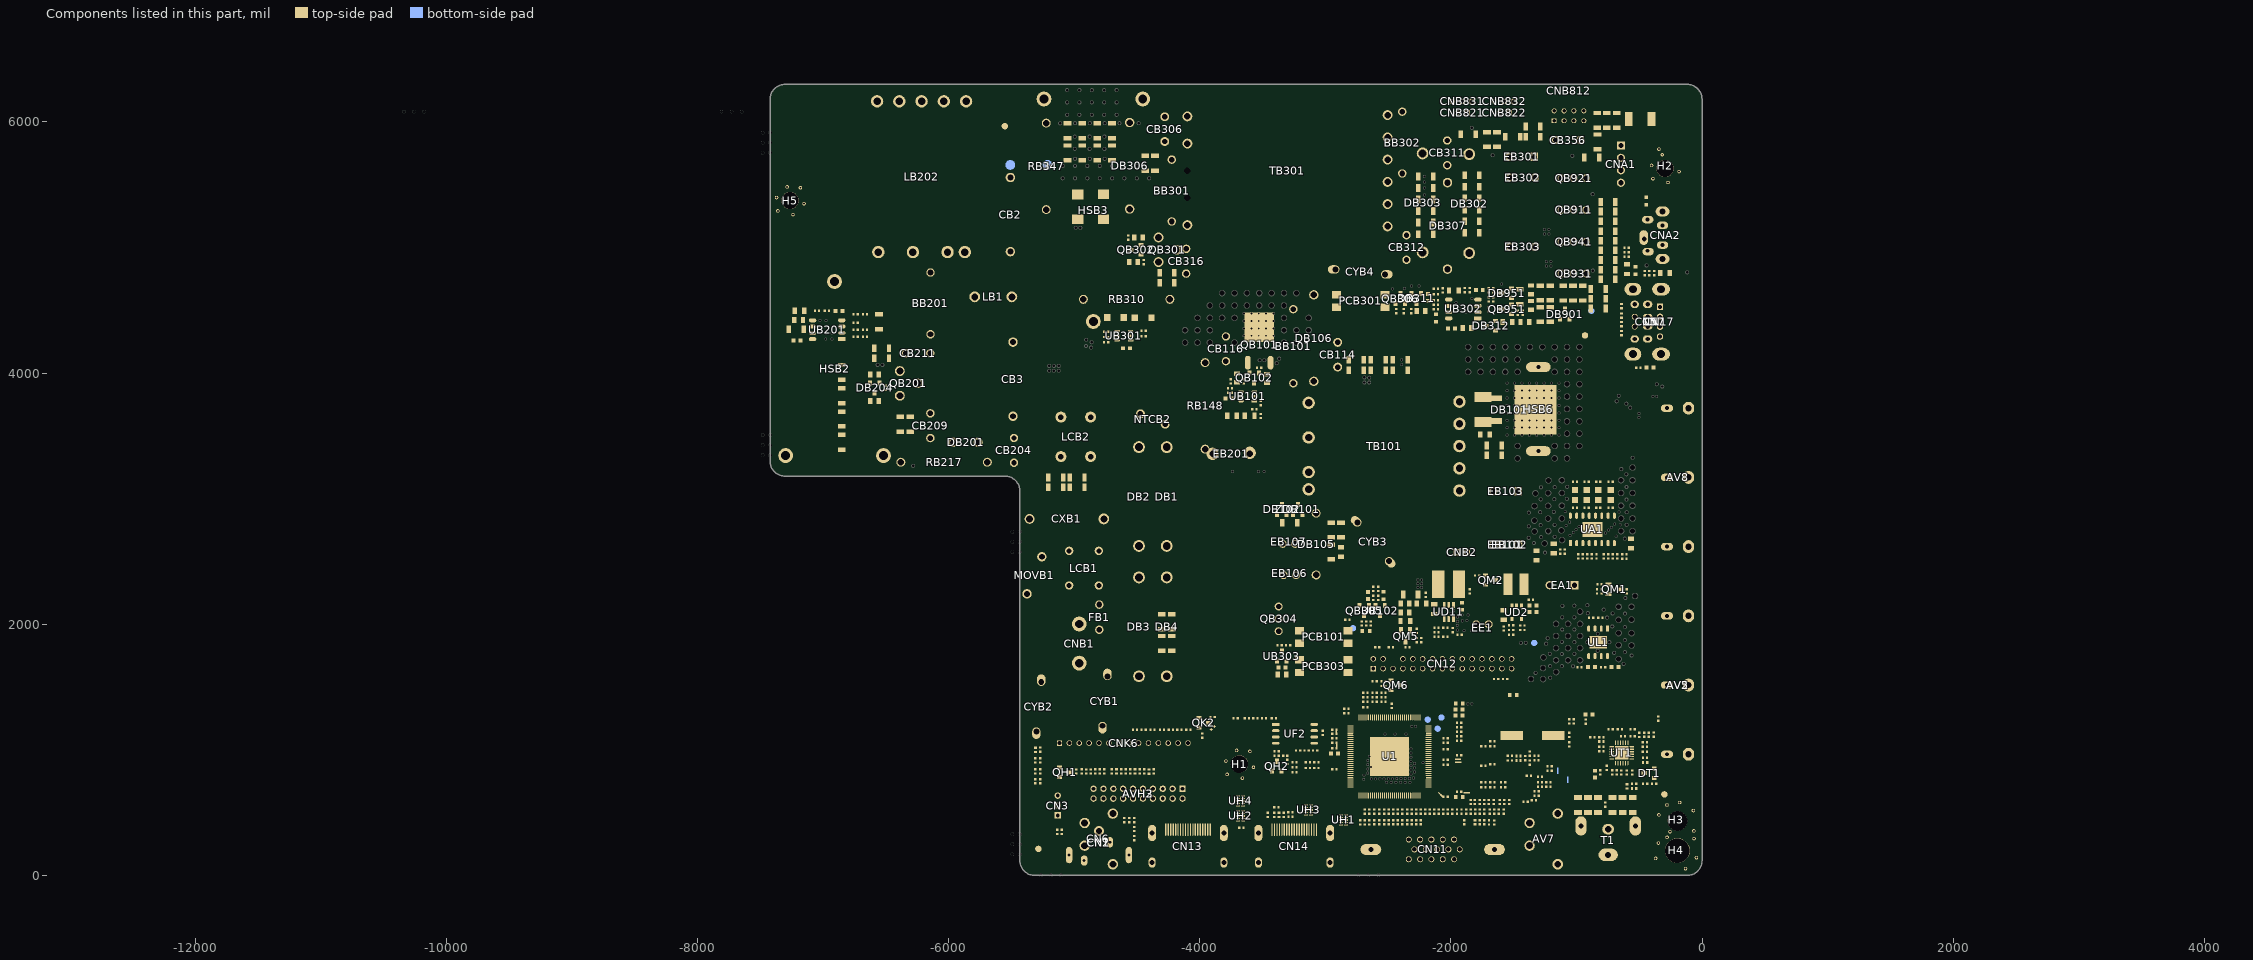
[diagram p0: the components of this part, seen from the top]
# Altium PCB MISC84277.PcbDoc (part 15 of 15)
Units mil, origin at the board's own origin, x right, y up, seen from the top; angles counter-clockwise.
Board outline 7422.08 x 6299.21 mil, 2 copper layers (TopLayer, BottomLayer), stack 61.855 mil thick; 709 components, 395 nets, 2812 pads, 811 vias.

## Silkscreen, mask and mechanical layers (free items; w line width, h text height)
TopOverlay:
  drawing of 481 lines, arcs and shapes, not listed
  text "LED DRIVER" at -855.43,6223.54 h60
  text "Solder Mask:" at 948.13,5998.57 h60
  text "IPC SM-840" at 1360.63,5997.57 h60
  text "Silkscreen Color:" at 2126.63,5997.57 h60
  text "White" at 2605.63,5997.57 h60
  text "Units:" at 2126.63,5898.57 h60
  text "PTH Copper Thickness:" at 948.13,5897.57 h60
  text "mm" at 2324.63,5897.07 h60
  text ">20um" at 1621.63,5896.57 h60
  text "4.2 --- 4.6" at 2127.29,5799.1 h60
  text "Dielectric Constant Er@1GHz To 1MHz:" at 947.79,5798.6 h60
  text "Panel Size:" at 946.13,5700.07 h60
  text "2L,2,164.00×165.50mm,FR4(TG130-CTI175),1OZ,Green,OSP,1.2mm" at 1251.29,5700.1 h60
  text "Silkscreen on PTH:" at 946.63,5598.57 h60
  text "Primary Side Retained;" at 1464.63,5597.57 h60
  text "Secondary Side  Removed for Soldering" at 2126.63,5596.07 h60
  text "Special Requirements" at 945.62,5507.89 h60
  text "If engineering questions get no reply within 2 hours, call: PHONE_A" at 2832.29,5500.6 h60
  text "SPEAKER" at -803.98,5452.5 h50 r90
  text "1. Lead-free hot air leveling (HAL_LF, Lead Free Hot Air Leveling)" at 1536.51,5404.3 h60
  text "2. Organic solderability preservative (OSP, Organic Solderability Preservatives)" at 1536.51,5320.3 h60
  text "3. Electroless nickel immersion gold (ENIG, Electroless Nickel/Immersion Gold)" at 1535.01,5228.8 h60
  text "Plated Technics" at 1020.63,5194.07 h60
  text "4. Electroless nickel immersion gold + gold finger (ENIG_G/F, Electroless Nickel/Immersion Gold + Gold Finger)" at 1536.51,5148.3 h60
  text "5. Gold plated (Gold_plated, Gold-plated)" at 1537.51,5067.8 h60
  text "6. Gold plated + gold finger (Gold_Plated_G/F, Gold-plated + Gold Finger)" at 1538.01,4989.8 h60
  text "Impedance Control" at 950.36,4761.21 h60
  text "Target Impedance" at 1747.19,4761.31 h60
  text "Width & Clearance" at 2493.02,4761.08 h60
  text "Layer(s)" at 3261.33,4761.39 h60
  text "75 +/- 10% Ohm" at 1769.39,4660.61 h60
  text "G/12/15.8/12/G mil" at 2450.44,4659.93 h60
  text "layer 1" at 3261.33,4660.05 h60
  text "Single End Impedance" at 950.36,4614.39 h60
  text "[ Zo ]" at 1173.86,4477.14 h60
  text "2" at -12847.94,4319.68 h160 r270
  text "G/5/7/5/7/5/G mil" at 2450.94,4263.43 h60
  text "100 +/- 10% Ohm" at 1746.89,4262.42 h60
  text "layer 1" at 3262.82,4260.64 h60
  text "Differential Impedance" at 950.22,4212.81 h60
  text "[ Zo ]" at 1173.35,4089.48 h60
  text "90 +/- 10% Ohm" at 1772.94,4064.43 h60
  text "layer 1" at 3258.82,4063.64 h60
  text "G/5/11/5/11/5/G mil" at 2450.94,4060.93 h60
  text "EXT-USB" at -281.5,4033.46 h60
  text "( G: Ground )" at 1083.43,3981.98 h60
  text "Common Mode Impedance" at 930,3760.3 h60
  text "[ Zc ]" at 1178,3679.3 h60
  text "Gerber Documents  .GTP&.GBP are used for making stencil" at 1842.55,3415.11 h60
  text "Stencil" at 943.42,3314.43 h60
  text "The same as XXXXXXXXXXXXX XXXXXX" at 1837.45,3222.78 h60
  text "Test jig" at 942.36,3122.45 h60
  text "The same as XXXXXXXXXXXXX XXXXXX" at 1838.45,3122.23 h60
  text "Wave-soldering jig" at 944.57,3024.21 h60
  text "The same as XXXXXXXXXXXXX XXXXXX" at 1840.35,3022.23 h60
  text "Solder paste" at 1842.55,2922.43 h60
  text "Production process" at 943.05,2920.93 h60
  text "Special Requirements" at 944.05,2822.93 h60
  text "Package Attention" at 943.43,2725.38 h60
  text "PWR UPGRADE" at -2224.9,2703.31 h60
  text "[Fragile components]" at 1179.66,2640.56 h60
  text "Footprint Matching" at 943.43,2525.38 h60
  text "GND" at -2144.95,2441.61 h50
  text "12V" at -1782,2438.93 h50
  text "[New component footprint]" at 1156.42,2437.43 h60
  text "Layer Stack Up Detail for" at 1084.39,2099.57 h100
  text ".Pcb_File_Name_No_Path" at 2145.21,2099.57 h100
  text "Layer" at 1248.75,1951.84 h50
  text "Gerber" at 1620.46,1951.84 h50
  text "Layer" at 1931.61,1951.84 h50
  text "Layer" at 2567.85,1951.84 h50
  text "Copper" at 3356.75,1951.84 h50
  text "Dielectric" at 3668.53,1951.84 h50
  text "Name" at 1248.75,1899.46 h50
  text "Document" at 1620.46,1899.46 h50
  text "Ordor" at 1931.61,1899.46 h50
  text "Stack up" at 2567.85,1899.46 h50
  text "Thickness" at 3356.75,1899.46 h50
  text "Height" at 3668.53,1899.46 h50
  text "1" at -67,1763 h160 r90
  text "TopOverlay" at 1248.45,1666.61 h60
  text ".GTO" at 1658.02,1664.05 h60
  text "T3.15AL 250V~" at -4651.2,1655.5 h78.74 r90
  text "0.4mil" at 3665.85,1579.02 h60
  text "LVDS" at -2202.76,1535.43 h60
  text "1" at 1984.81,1475.87 h60
  text "1.4mil" at 3369.81,1475.81 h60
  text "2" at 1984.87,1262.83 h60
  text "1.4mil" at 3368.1,1261.82 h60
  text "0.4mil" at 3668.52,1167.14 h60
  text "IR&KEY" at -4140.7,871.8 h60
  text "Notes:" at 920.32,604.26 h80
  text "1. No Plated Through Hole  overlap each other should be combined ,Residues between them should be eliminated." at 919.45,516.35 h60
  text "EXT-HDMI" at -4407.2,458 h55
  text "EXT-LINE OUT" at -4961,448.8 h55 r90
  text "2. Plated Through Hole superposition should be made as a bigger one." at 919.39,440.25 h60
  text "3. When there is not enough space for UL authentication marking,Manufacturer ID code and the Bar Code frame," at 919.45,371.75 h60
  text "only the Manufacturer  ID code is needed and layed wherever it can be." at 977.83,301.06 h60
  text "4. Spacing between two pads of IC package should be covered with solder oil." at 919.45,224.29 h60
  text "5. All trace should be covered with green oil unless otherwise specified. If discovers unusually, please confirm with us." at 919.45,150.88 h60
  text "6. Silkscreen overlaped SMD pads should be removed directly." at 919.45,77.57 h60
  text "7. The width of Carbon Sprayed must be 16mil wider than its trace." at 919.45,6.53 h60
  text "8. Bridging Thickness of V-cut  should be kept within 0.3±0.1mm when the width of single piece bare board is smaller than 20mm." at 919.45,-67.9 h60
  text "9. There is no need to plugged with green oil when the diameter of vias is bigger than 0.6mm." at 919.45,-149.73 h60
  text "10. All vias under BGA must be covered and plugged with green oil." at 919.46,-229.6 h60
BottomOverlay:
  circle w4: c-4654.25,2250.38 r2
  circle w5.91: c-4654.25,2205.01 r2
  circle w5.91: c-4881.89,3062.9 r2
  circle w4: c-4881.89,3108.27 r2
  circle w5.91: c-4881.89,3153.45 r2
  circle w4: c-4881.89,3198.82 r2
  circle w5.91: c-5240.16,3062.9 r2
  circle w4: c-5240.16,3108.27 r2
  circle w5.91: c-5240.16,3151.48 r2
  circle w4: c-5240.16,3196.85 r2
  rectangle: 1083.01,1048.5 1213.21,1127.24
  lines w5: -5241.67,3108.25 -5240.16,3076.77 -5238.65,3108.25 ; -5241.67,3196.83 -5240.16,3165.35 -5238.65,3196.83 ; -5092.4,439.8 -5083.4,448.8 -4950.9,448.8 -4950.9,671.4 -5092,671.4 ; -4883.4,3108.25 -4881.89,3076.77 -4880.38,3108.25 ; -4883.4,3198.8 -4881.89,3167.32 -4880.38,3198.8 ; -4655.76,2250.36 -4654.25,2218.89 -4652.74,2250.36 ; -2027.41,6201.04 -2027.41,6271.65 -1795.11,6271.65 -1795.11,6202.51 ; -1996.14,6017.15 -1996.14,5954.72 -1821.14,5954.72 -1821.14,6017.15 ; -1692.13,6201.04 -1692.13,6271.65 -1459.83,6271.65 -1459.83,6202.51 ; -1660.87,6017.15 -1660.87,5954.72 -1485.87,5954.72 -1485.87,6017.15 ; -1224.05,6114.37 -1224.05,6267.72 -894.05,6267.72 -894.05,6119.37 ; -301.58,4252.69 -129.92,4252.69 -129.92,4564.32 -298.27,4564.32 ; 1633.91,1048.5 1633.91,1127.24 ; -5292.98,3051.45 -5239.83,3128.22 -5190.62,3051.45 -5292.98,3051.45 ; -5292.98,3140.03 -5239.83,3216.8 -5190.62,3140.03 -5292.98,3140.03 ; -4934.72,3051.45 -4881.57,3128.22 -4832.35,3051.45 -4934.72,3051.45 ; -4934.72,3142 -4881.57,3218.77 -4832.35,3142 -4934.72,3142 ; -4707.08,2193.57 -4604.71,2193.57 -4653.93,2270.34 -4707.08,2193.57 ; -759.2,1208.67 -347.06,1208.67 -347.06,1661.42 -759.2,1661.42 -759.2,1208.67 ; 1083.01,1048.5 1815.04,1048.5 1815.04,1127.24 1083.01,1127.24 1083.01,1048.5
  lines w8: -5060.4,863.1 -4044.32,863.1 -4044.32,1079.8 ; -696,5467.46 -696,5863.17 -493.9,5863.17 -493.9,5467.46 -696,5467.46
  text "NC" at -1147.64,6222.44 h51.18
  text "NC" at -1070.87,6222.44 h51.18
  text "GND" at -908.33,6222.44 h50
  text "NC" at -1881.1,6217.88 h51.18
  text "NC" at -1545.82,6217.88 h51.18
  text "-" at -1022.5,6212.6 h118.11
  text "+" at -1810.75,6209.46 h78.74
  text "+" at -1475.47,6209.46 h78.74
  text "-" at -1975.89,6206.86 h118.11
  text "-" at -1640.61,6206.86 h118.11
  text "NC" at -1151.57,6161.42 h51.18
  text "NC" at -1070.87,6161.42 h51.18
  text "GND" at -909.45,6161.42 h50
  text "-" at -1019.69,6149.61 h118.11
  text "-" at -1936.52,5960.79 h118.11
  text "-" at -1601.24,5960.79 h118.11
  text "+" at -1852.09,5959.46 h78.74
  text "+" at -1516.81,5959.46 h78.74
  text "ROUT+" at -545.1,5708 h50 r270
  text "ROUT-" at -595,5650.8 h50 r270
  text "LOUT-" at -545.1,5540.5 h50 r270
  text "LOUT+" at -595,5481.8 h50 r270
  text "EAPHONE OUT" at -66.22,4906.05 h60 r270
  text "USB" at -103.5,4350.3 h60 r270
  text "CVBS OUT&AUDIO IN/AV2 IN" at -200,2571 h60 r270
  text "FB1" at -4630.8,2148.5 h48.31
  text "T3.15AL 250V~" at -4697.1,1655.5 h78.74 r270
  text ".GBO" at 1658.64,1071.53 h60
  text "BottomOverlay" at 1236.97,1070.54 h60
  text "YPBPR/AV1 IN" at -196,1054 h60 r270
  text "K3/V+" at -4736.25,874.5 h50 r270
  text "NC" at -4997.9,873.2 h50 r270
  text "K6/P" at -4956.1,872.9 h50 r270
  text "K5/M" at -4893.79,873.5 h50 r270
  text "K4/V-" at -4814.98,873.5 h50 r270
  text "K2/C-" at -4657.44,873.5 h50 r270
  text "K1/C+" at -4578.67,873.5 h50 r270
  text "K0/S" at -4499.95,872.5 h50 r270
  text "GND" at -4421.18,872.5 h50 r270
  text "IR" at -4342.44,872.5 h50 r270
  text "GND" at -5037.9,871.1 h50 r270
  text "GRN" at -4263.64,871.5 h50 r270
  text "RED" at -4184.29,871.5 h50 r270
  text "5V" at -4106.1,871.5 h50 r270
  text "IR" at -4340.03,740 h50 r270
  text "L" at -5025,622.8 h50
  text "GND" at -4962.4,540.5 h50
  text "R" at -5007.5,464.3 h50
  text "AV1 IN/AV OUT" at -4601.9,233.7 h50 r270
  text "COAX/CVBS OUT" at -4645.9,190.3 h50 r270
  text "VGA IN" at -2469,50 h60
  text "HDMI 2" at -2729,49 h60
  text "PC AUDIO IN" at -1223,49 h60
  text "RF IN" at -694,46 h60
  text "HDMI 1(ARC)" at -3740,22 h60 r270
TopPaste:
  drawing of 42 lines, arcs and shapes, not listed
  text "TopPaste" at 1248.45,1763.14 h60
  text ".GTP" at 1658.02,1761.01 h60
BottomPaste:
  rectangle: 1083.01,954.35 1213.21,1033.09
  lines w5: 1633.91,954.35 1633.91,1033.09 ; 1083.01,954.35 1083.01,1033.09 1815.04,1033.09 1815.04,954.35 1083.01,954.35
  text "BottomPaste" at 1235.81,977.33 h60
  text ".GBP" at 1658.91,972.21 h60
TopSolder:
  drawing of 42 lines, arcs and shapes, not listed
  text "TopSolder" at 1248.95,1572.06 h60
  text ".GTS" at 1658.02,1570.41 h60
BottomSolder:
  drawing of 58 lines, arcs and shapes, not listed
  text "BottomSolder" at 1235.81,1163.74 h60
  text ".GBS" at 1657.99,1162.85 h60
过炉治具:
  drawing of 272 lines, arcs and shapes, not listed
3D和装配:
  circle w10: c-196.85,5708.82 r233.11
  circle w10: c-295.28,5629.92 r233.11
  lines w5: -118.47,6299.21 -0.37,6299.21 -0.37,6181.1 ; 0,5727.78 0,5845.89
  lines w82.68: -5611.2,3517.2 -5611.2,3806 -5460.2,3957 -5452,3957 -5487,3922 ; -5264.3,4090.6 -5264.3,3999.7 -5218.2,3953.6 -4683.2,3953.6 ; -5258.57,4183.3 -5155.3,4183.3 -5058.1,4086.1 ; -5243.35,4059.38 -5140.19,4059.38 ; -5226.7,4404.29 -5226.7,4507.45 ; -5223.67,3864.5 -5120.5,3864.5 ; -5183.07,4190.94 -5079.91,4190.94 ; -5183.07,4240 -5034.5,4240 -4936.6,4142.1 -4603.7,4142.1 ; -3518.52,4179.13 -3415.35,4179.13 ; -3335.45,4795.28 -3232.28,4795.28 ; -3086.73,4807.2 -3013.78,4734.25 ; -3004.65,4509.98 -3004.65,4613.14
  lines w118.11: -5317.8,2431.6 -5226.8,2431.6 -5148.59,2509.81 -5148.59,2612.11 -5051.6,2709.1 -4983.6,2709.1 ; -5307.1,2741.7 -5228.66,2820.14 ; -5073.53,2004.47 -5020.5,2057.5 ; -4919.47,3766.3 -4816.3,3766.3 ; -4894.67,3693.5 -4791.5,3693.5 ; -4514.87,3281.21 -4605.5,3371.83 -4605.5,3475 -4605.5,3376.2 -4512.69,3283.39 ; -4594.4,2325.9 -4545.5,2277 -4594.4,2325.9 ; -4594.4,2325.9 -4594.4,2436.83 -4594.4,2325.9
  lines w125.98: -4839.4,1783.3 -4871.3,1815.2 -4995.9,1815.2 -5100.3,1919.6 -5100.3,2037.09 -5000.45,2136.94 -4923.02,2136.94 -4840.98,2054.9 -4789.5,2054.9
  lines w157.48: -3409.45,3627.95 -3409.45,3731.12
顶层限制:
  drawing of 4184 lines, arcs and shapes, not listed
  text "11.2" at 3482.53,5302.97 h98.43 r180
  text "6.5" at 2304.6,5197.25 h98.43 r166
  text "7" at 3242.66,4998.08 h98.43 r180
  text "0.5" at 3361.73,4692.28 h98.43 r180
  text "GND" at -341.53,4586.36 h50 r90
  text "DP" at -341.53,4472.25 h50 r90
  text "DM" at -341.53,4393.94 h50 r90
  text "5V" at -341.53,4302.74 h50 r90
  text "14.4" at 2602.87,4263.67 h98.43 r90
  text "15.0" at 2255.02,4246.94 h98.43 r90
  text "7.0" at 3364.47,4230.17 h98.43 r180
  text "16.0" at 3513.3,4204.84 h98.43 r180
  text "9.5" at 3333.16,3915.29 h98.43 r180
  text "AC IN" at -6814.98,3707.33 h157.48
  text "14" at 460.2,3374.68 h98.43 r90
  text "3- 8.3" at 3581.8,3151.3 h98.43 r150
  text "40.2" at 2411.04,3012.29 h98.43 r90
  text "14" at 461.94,2823.49 h98.43 r90
  text "5.5" at 3327.04,2566.95 h98.43 r180
  text "9.5" at 3333.16,2261.75 h98.43 r180
  text "14" at 460.2,1721.13 h98.43 r90
  text "3- 8.3" at 3581.8,1497.76 h98.43 r150
  text "LVDS" at -2391.73,1424.67 h157.48
  text "40.2" at 2411.04,1358.75 h98.43 r90
  text "14" at 461.94,1169.95 h98.43 r90
  text "IR&KEY" at -4849.28,1115.47 h157.48
  text "14" at 3418.6,915.94 h157.48 r90
  text "5.5" at 3327.04,913.41 h98.43 r180
  text "7    8    9   10   11   12    13    15" at 4400.83,906.2 h157.48 r90
  text "1.2" at 3323.22,-119.3 h98.43
  text "5.2" at -2507.19,-440.39 h98.43
  text "25" at -2228.32,-2181.44 h98.43
  text "11.2" at -923.4,-2197.98 h98.43
  text "6" at -4732.6,-2212.45 h98.43 r66
  text "6" at -1492.87,-2238.08 h98.43
  text "8.3" at -4689.87,-2323.86 h98.43 r56
  text "8.3" at -4689.87,-2323.86 h98.43 r56
  text "7" at -1271.95,-2333.1 h98.43
  text "10.25" at -4913.59,-2358.45 h98.43 r90
  text "10.25" at -4913.59,-2358.45 h98.43 r90
  text "15" at -4168.06,-2492.43 h98.43
  text "15" at -3321.61,-2492.43 h98.43
  text "6.3" at -632.4,-2832.36 h98.43 r270
  text "7" at -1146.61,-2938.1 h98.43 r90
  text "5.5" at -4842.59,-2978.1 h98.43
  text "5.5" at -4842.59,-2978.1 h98.43
  text "16.3" at -2323.99,-3063.33 h98.43
  text "7" at -4655.52,-3082.1 h98.43 r90
  text "9.3" at -4841.19,-3150.74 h98.43 r90
  text "6.3" at -1523.2,-3248.76 h98.43 r90
  text "7.9" at -1654.31,-3249.94 h98.43 r90
  text "0.7" at -3781.68,-3294.43 h98.43 r90
  text "0.7" at -2935.22,-3294.43 h98.43 r90
  text "5.6" at -4304.24,-3297.05 h98.43 r90
  text "5.6" at -3457.78,-3297.05 h98.43 r90
  text "12.6" at -2537.98,-3298.53 h98.43 r90
  text "1      2      3         4       5    6" at -4884.66,-3647.41 h157.48
底层限制:
  circle w5: c-5312.1,562.78 r98.43
附加说明:
  lines w5: 2080.94,6270.26 3565.94,6270.26 ; 2080.94,6377.6 3565.94,6377.6 ; 2080.94,6484.93 3565.94,6484.93 ; 2080.94,6592.26 3565.94,6592.26 ; 2080.94,6699.6 4060.94,6699.6 ; 2575.94,6162.93 2575.94,6806.93 ; 3070.94,6162.93 3070.94,6806.93 ; 3565.94,6162.93 3565.94,6806.93 ; 2080.94,6162.93 2080.94,6806.93 4060.94,6806.93 4060.94,6162.93 2080.94,6162.93
  text "TV designer" at 2692.94,6735.93 h60
  text "Power designer" at 3191.94,6735.93 h60
  text "Customer" at 3756.44,6735.43 h60
  text "Version / cycle no." at 2198.44,6731.43 h60
  text "A16XXX" at 2199.44,6626.43 h60
  text "XXXXXX" at 2194.44,6520.13 h60
  text "LJJ" at 2754.5,6520 h60
  text "SY" at 3760.44,6447.23 h60
  text "XXXXXX" at 2202.44,6413.03 h60
  text "CXJ" at 2758.47,6413.03 h60
  text "ZCL" at 3271.34,6413.03 h60
  text "XXXXXX" at 2203.14,6302.73 h60
  text "CK" at 2758.97,6296.63 h60
  text "Utilization:" at 2845.63,6000.57 h60
  text "73%" at 3164.13,6000.57 h60
  text "Via/Pad/Slot Holes(Unit Area):" at 2844.79,5901.1 h60
  text "0.XX/mm²" at 3652.29,5897.1 h60
  text "2016.03.31" at 3739.63,5602.07 h60
  text "Special requirements; leave blank if none" at 1549.95,5499.44 h60
  text "Customer special requirements; special process requirements; leave blank if none" at 1840.32,2823.64 h60
  text "Fragile component designators; leave blank if none" at 1838.55,2677.48 h60
  text "New footprint designators; leave blank if none" at 1840.92,2470.43 h60
  text "X.XXXX.XXX Manufacture Information" at 922.22,-319.04 h60
  text "Pick Place for  X.XXXX.XXX" at 922.22,-391.75 h60
  text "X.XXXX.XXX Gerber files for Stencil" at 921.79,-463.9 h60
  text "X.XXXX.XXX PCB Layout for Authentication_A0" at 920.79,-540.9 h60
  text "X.XXXX.XXX repair PCB_A0" at 922.29,-619.4 h60
  text "X.XXXX.XXX Silkscreen" at 922.79,-696.4 h60
  text "X.XXXX.XXX Stencil Revision Explanation" at 922.79,-764.9 h60
  text "X.XXXX.XXX Testing jig Revision Explanation" at 922.29,-833.9 h60
  text "X.XXXX.XXX Wave-soldering jig Revision Explanation" at 921.79,-901.9 h60
  text "X.XXXX.XXX Bonding Explanation" at 919.22,-975.69 h60
DrillDrawing:
  text ".Legend" at 922.61,6117.32 h60